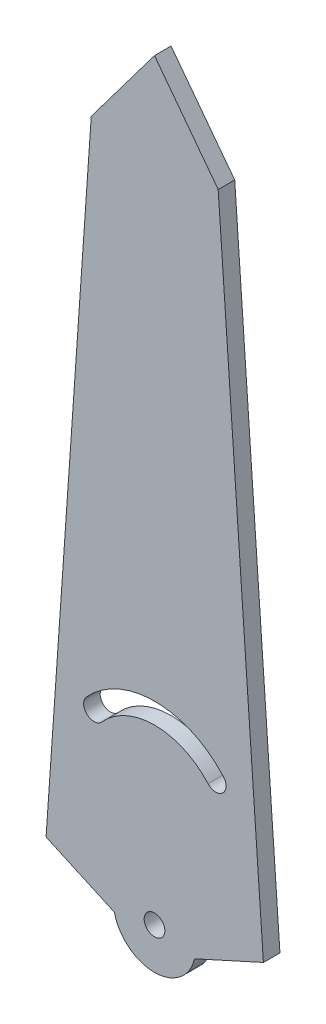
from build123d import *

# Parameters (mm, degrees)
SKETCH2_R           = 5
BOSS_EXTRUDE1_DEPTH = 8
CUT_EXTRUDE1_DEPTH  = 10


with BuildPart() as part:
    # Sketch2 → Boss-Extrude1 (new body)
    with BuildSketch(Plane.XY):
        with BuildLine():
            Line((52.661413708, 1194.6), (30.792715617, 1507.336952872))
            Line((30.792715617, 1507.336952872), (0, 1548.052221237))
            Line((0, 1548.052221237), (-30.569888201, 1507.336952872))
            Line((-30.569888201, 1507.336952872), (-52.438586292, 1194.6))
            Line((-52.438586292, 1194.6), (-19.401690748, 1179.61379954))
            ThreePointArc((-19.401690748, 1179.61379954), (-0.057863528, 1164.108770521), (19.375843714, 1179.500995806))
            Line((19.375843714, 1179.500995806), (52.661413708, 1194.6))
        make_face()
        with Locations((0, 1184)):
            Circle(SKETCH2_R, mode=Mode.SUBTRACT)
    extrude(amount=BOSS_EXTRUDE1_DEPTH)

    # Sketch3 → Cut-Extrude1 (cut)
    with BuildSketch(Plane.XY.offset(8)):
        with BuildLine():
            ThreePointArc((33.346114696, 1262.714191316), (0.208267219, 1277.711712086), (-32.994808317, 1262.859158782))
            ThreePointArc((-32.994808317, 1262.859158782), (-32.584628739, 1255.799997875), (-25.525467832, 1256.210177452))
            ThreePointArc((-25.525467832, 1256.210177452), (0.186415379, 1267.711735961), (25.847787119, 1256.097917173))
            ThreePointArc((25.847787119, 1256.097917173), (32.905087979, 1255.656890456), (33.346114696, 1262.714191316))
        make_face()
    extrude(amount=-CUT_EXTRUDE1_DEPTH, mode=Mode.SUBTRACT)


solid = part.part
